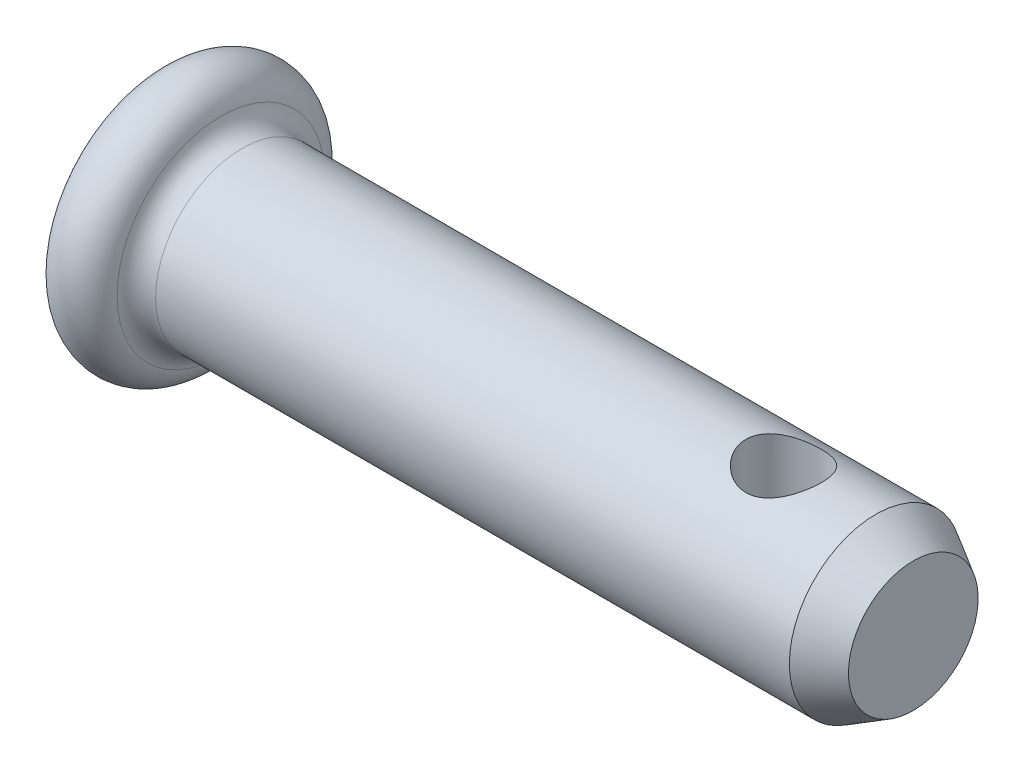
from build123d import *

# Parameters (mm, degrees)
FILLET_1_R          = 0.5
CHAMFER_1_SIZE      = 0.866025404
CHAMFER_1_SIZE2     = 0.5
SKETCH_2_R          = 0.87
CUT_EXTRUDE_1_DEPTH = 500


with BuildPart() as part:
    # 草图1 → Revolve 700 (revolve)
    with BuildSketch(Plane.XY, mode=Mode.PRIVATE) as revolve_700_sk:
        with BuildLine():
            Line((0, 0), (17.5, 0))
            Line((17.5, 0), (17.5, 2))
            Line((17.5, 2), (1.5, 2))
            Line((1.5, 2), (1.5, 2.25))
            ThreePointArc((1.5, 2.25), (0.75, 3), (0, 2.25))
            Line((0, 2.25), (0, 0))
        make_face()
    revolve(revolve_700_sk.sketch.rotate(Axis((0, 0, 0), (1, 0, 0)), 90), axis=Axis((0, 0, 0), (1, 0, 0)))

    # 圆角1
    fillet_1_edges = [part.edges().sort_by_distance(p)[0] for p in [
        (1.5, 0, -2),
    ]]
    fillet(fillet_1_edges, radius=FILLET_1_R)

    # 倒角1
    chamfer_1_edges = [part.edges().sort_by_distance(p)[0] for p in [
        (17.5, 0, -2),
    ]]
    chamfer_1_side = [part.faces().sort_by_distance(p)[0] for p in [
        (9.737372436, 0, -2),
    ]]
    chamfer(chamfer_1_edges, length=CHAMFER_1_SIZE, length2=CHAMFER_1_SIZE2, reference=chamfer_1_side[0])

    # 草图2 → 切除-拉伸1 (cut, symmetric)
    with BuildSketch(Plane(origin=(0, 0, 0), x_dir=(1, 0, 0), z_dir=(0, 1, 0))):
        with Locations(Location((14.5, 0, 0), (0, 0, 270))):
            Circle(SKETCH_2_R)
    extrude(amount=CUT_EXTRUDE_1_DEPTH, both=True, mode=Mode.SUBTRACT)


solid = part.part
